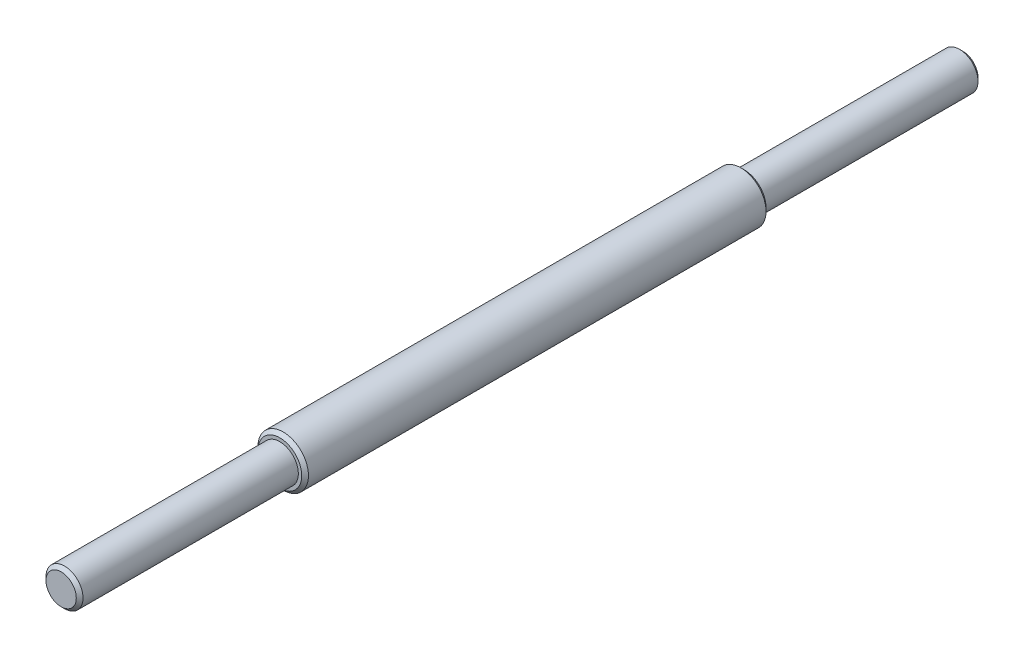
SolidWorks part; units mm, degrees
ref_plane "Front Plane" through (0, 0, 0) normal (0, 0, 1) x (1, 0, 0)
ref_plane "Top Plane" through (0, 0, 0) normal (0, 1, 0) x (1, 0, 0)
ref_plane "Right Plane" through (0, 0, 0) normal (1, 0, 0) x (0, 0, -1)
sketch "Sketch1" plane through (0, 0, 0) normal (0, 0, 1) x (1, 0, 0)
  circle A0 centre (0, 0) radius 7.5
  dimension "D1" = 15
extrude "Boss-Extrude1" add sketch "Sketch1" along normal blind 138
sketch "Sketch2" plane through (0, 0, 138) normal (0, 0, 1) x (1, 0, 0)
  circle A0 centre (0, 0) radius 5.5
  dimension "D1" = 11
extrude "Boss-Extrude2" add sketch "Sketch2" along normal blind 20
sketch "Sketch3" plane through (0, 0, 158) normal (0, 0, 1) x (1, 0, 0)
  circle A0 centre (0, 0) radius 5.5
  dimension "D1" = 11
extrude "Boss-Extrude3" add sketch "Sketch3" along normal blind 45
chamfer "Chamfer1" distance 1 angle 45 3 edges at (5.5, 0, 203) (7.5, 0, 0) (7.5, 0, 138)
sketch "Sketch4" plane through (0, 0, 0) normal (0, 0, -1) x (-1, 0, 0)
  circle A0 centre (0, 0) radius 5.5
  dimension "D1" = 11
extrude "Boss-Extrude4" add sketch "Sketch4" along normal blind 65
chamfer "Chamfer2" distance 1 angle 45 1 edges at (-5.5, 0, -65)
